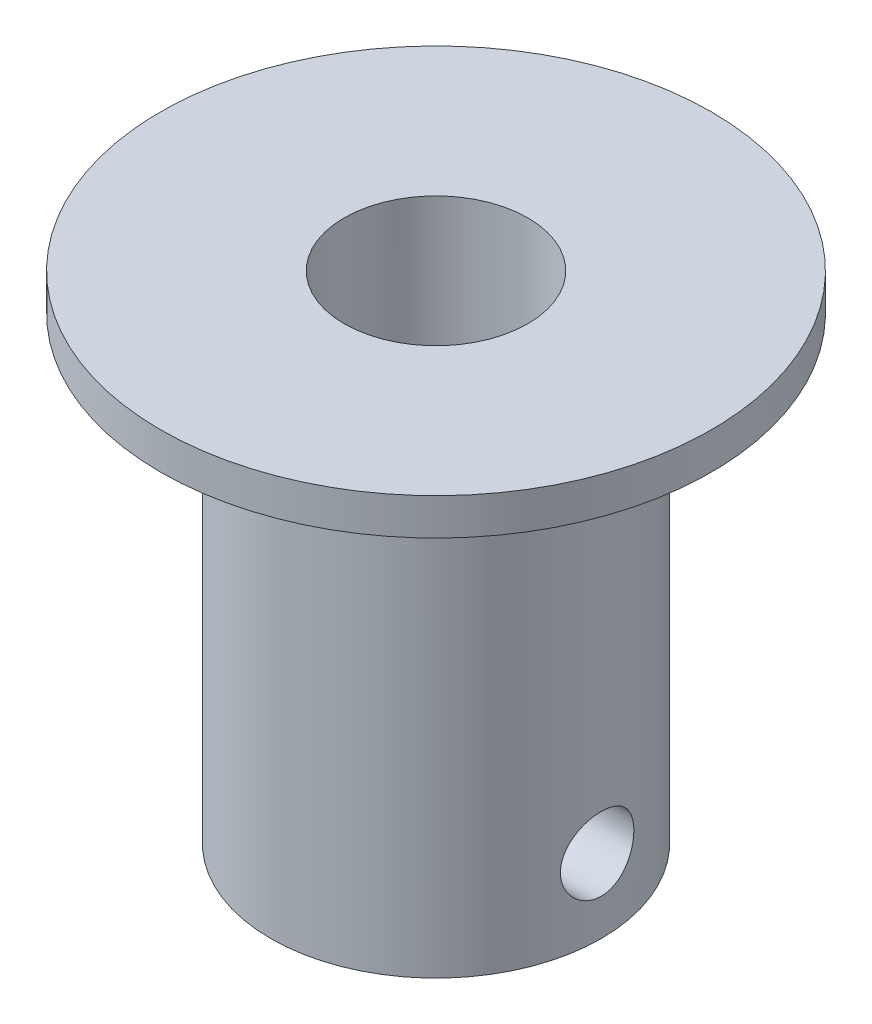
from build123d import *
from build123d.topology import SkipClean

# Parameters (mm, degrees)
SKETCH2_R               = 75
SKETCH2_R_2             = 25
BOSS_EXTRUDE1_DEPTH     = 10
BOSS_EXTRUDE2_START     = 125
SKETCH3_R               = 45
SKETCH3_R_2             = 25
BOSS_EXTRUDE2_DEPTH     = 125
CUT_EXTRUDE1_DEPTH      = 164.935963108
CUT_EXTRUDE1_DEPTH_BACK = 164.935963108
SKETCH4_R               = 10


with BuildPart() as part:
    # Sketch2 → Boss-Extrude1 (new body)
    with BuildSketch(Plane(origin=(0, 0, 0), x_dir=(1, 0, 0), z_dir=(0, 1, 0))):
        with Locations(Location((0, 0, 0), (0, 0, 270))):
            Circle(SKETCH2_R)
        with Locations(Location((0, 0, 0), (0, 0, 270))):
            Circle(SKETCH2_R_2, mode=Mode.SUBTRACT)
    extrude(amount=BOSS_EXTRUDE1_DEPTH)

    # Sketch3 → Boss-Extrude2 (add)
    with SkipClean():  # the faces are left unmerged after this step: merging them gives an invalid solid
        with BuildSketch(Plane.XZ.offset(BOSS_EXTRUDE2_START)):
            with Locations(Location((0, 0, 0), (0, 0, 90))):
                Circle(SKETCH3_R)
            with Locations(Location((0, 0, 0), (0, 0, 270))):
                Circle(SKETCH3_R_2, mode=Mode.SUBTRACT)
        extrude(amount=-BOSS_EXTRUDE2_DEPTH)

    # Sketch4 → Cut-Extrude1 (cut, two sides: drawn at the far end of the back side and taken through both)
    with SkipClean():  # the faces are left unmerged after this step: merging them gives an invalid solid
        with BuildSketch(Plane(origin=(0, 0, 0), x_dir=(0, 0, -1), z_dir=(1, 0, 0)).offset(-CUT_EXTRUDE1_DEPTH_BACK)):
            with Locations((0, -105)):
                Circle(SKETCH4_R)
        extrude(amount=CUT_EXTRUDE1_DEPTH + CUT_EXTRUDE1_DEPTH_BACK, mode=Mode.SUBTRACT)


solid = part.part
